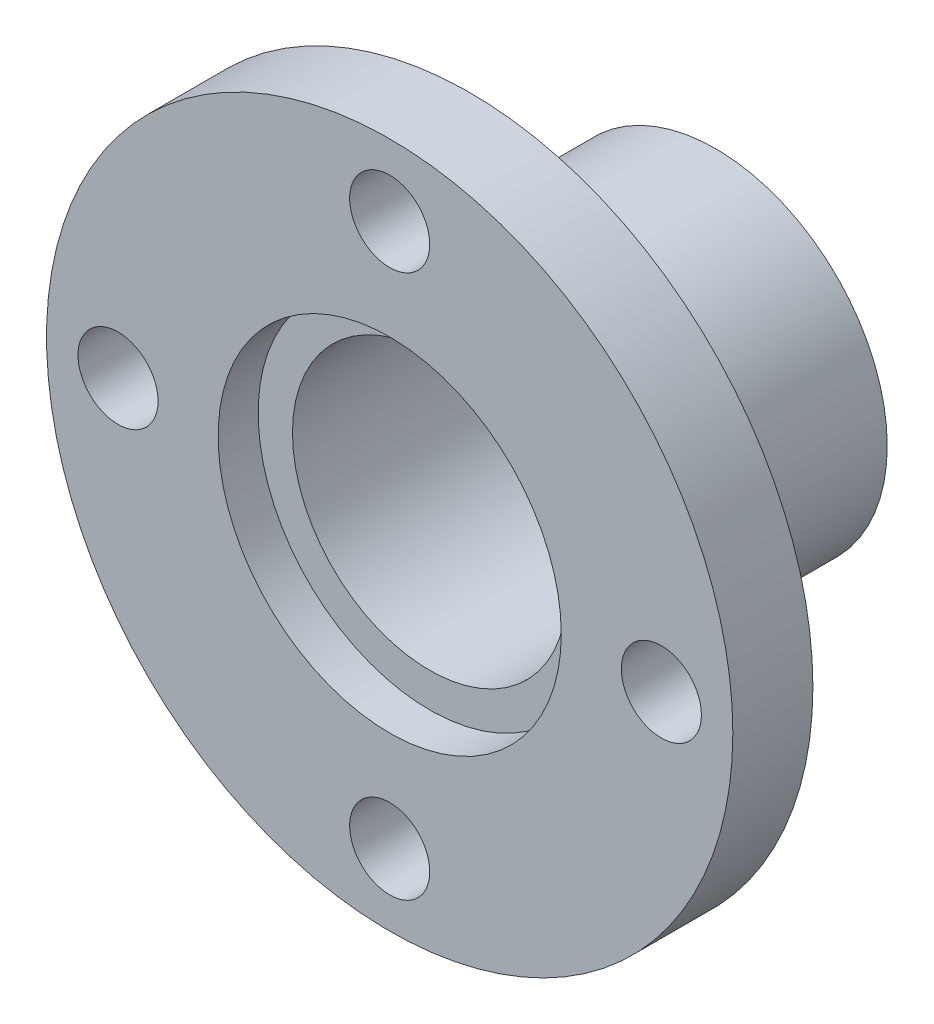
SolidWorks part; units mm, degrees
material "K"
ref_plane "Front" through (0, 0, 0) normal (0, 0, 1) x (1, 0, 0)
ref_plane "Top" through (0, 0, 0) normal (0, 1, 0) x (1, 0, 0)
ref_plane "Right" through (0, 0, 0) normal (1, 0, 0) x (0, 0, -1)
sketch "Sketch1" plane through (0, 0, 0) normal (0, 0, 1) x (1, 0, 0)
  circle A0 centre (0, 0) radius 24
  dimension "D1" = 48
extrude "Extrude-Thin1" add sketch "Sketch1" along normal blind 50 thin
sketch "Sketch2" plane through (0, 0, 50) normal (0, 0, 1) x (1, 0, 0)
  circle A0 centre (0, 0) radius 60
  circle A1 centre (0, 0) radius 30
  dimension "D1" = 120
extrude "Boss-Extrude1" add sketch "Sketch2" along normal mid plane 14 separate body
sketch "Sketch3" plane through (0, 0, 57) normal (0, 0, 1) x (1, 0, 0)
  circle A0 centre (0, 0) radius 47.5 construction
  dimension "D1" = 95
hole_wizard "Ø14.0 (14) Diameter Hole1" positions "Sketch6" profile "Sketch4" hole size "Ø14.0" standard "GB" end condition up to next
sketch "Sketch6" plane through (0, 0, 57) normal (0, 0, 1) x (1, 0, 0)
  circle A0 centre (0, 0) radius 47.5 construction
  point P0 (0, 47.5)
  point P4 (-47.5, 0)
  point P6 (47.5, 0)
  point P8 (0, -47.5)
sketch "Sketch4" plane through (0, 47.5, 57) normal (1, 0, 0) x (0, -1, 0)
  line L0 (0, 0) -> (0, 14.001)
  line L1 (0, 14.001) -> (7, 14.001)
  line L2 (7, 14.001) -> (7, 0)
  line L5 (7, 0) -> (0, 0)
  line L11 (0, -6.35) -> (0, 107.95) construction
  dimension "通孔孔直径" = 14
  dimension "通孔孔深度" = 14.001
sketch "Sketch7" plane through (0, 0, 0) normal (0, 0, -1) x (-1, 0, 0)
  point P0 (0, 0)
equation "\"零件重量\"= IIF ( \"SW-质量\" > 100 , int ( \"SW-质量\" ) , \"SW-质量\" )"
